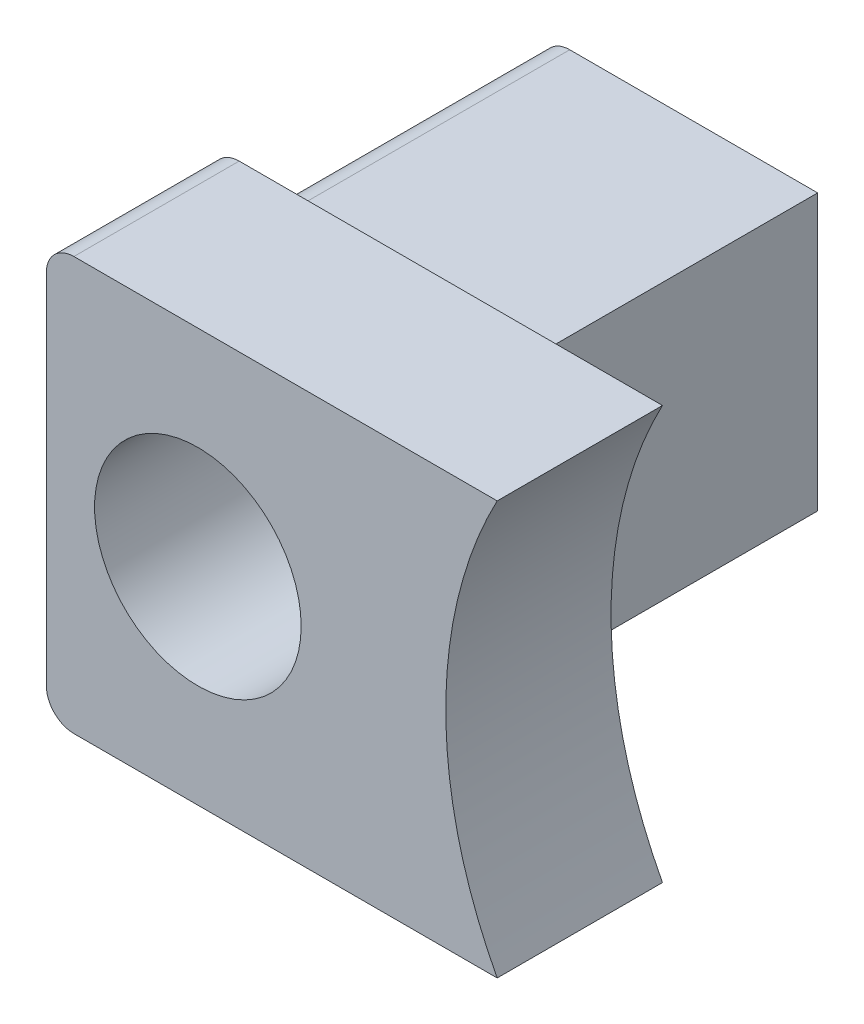
SolidWorks part; units mm, degrees
ref_plane "Front Plane" through (0, 0, 0) normal (0, 0, 1) x (1, 0, 0)
ref_plane "Top Plane" through (0, 0, 0) normal (0, 1, 0) x (1, 0, 0)
ref_plane "Right Plane" through (0, 0, 0) normal (1, 0, 0) x (0, 0, -1)
sketch "Sketch1" plane through (0, 0, 0) normal (0, 0, 1) x (1, 0, 0)
  line L1 (-8.25, 7.5) -> (8.25, 7.5)
  line L2 (-8.25, 7.5) -> (-8.25, -7.5)
  line L3 (-8.25, -7.5) -> (8.25, -7.5)
  line L4 (8.25, 7.5) -> (8.25, -7.5)
  line L5 (-8.25, 7.5) -> (8.25, -7.5) construction
  line L6 (-8.25, -7.5) -> (8.25, 7.5) construction
  point P0 (0, 0)
  dimension "D1" = 16.5
  dimension "D2" = 15
extrude "Boss-Extrude1" add sketch "Sketch1" along normal blind 18
fillet "Fillet1" radius 1 2 edges at (-8.25, -7.5, 9) (-8.25, 7.5, 9)
hole_wizard "CBORE for M4 Hex Socket Head Cap Screw1" positions "Sketch2" profile "Sketch3" counterbore size "M4" standard "ISO" end condition up to next
sketch "Sketch2" plane through (0, 0, 18) normal (0, 0, 1) x (1, 0, 0)
  line L0 (-8.25, 6.5) -> (-8.25, -6.5) construction
  point P0 (-2.75, 0)
  dimension "D1" = 5.5
sketch "Sketch3" plane through (-2.75, 0, 18) normal (1, 0, 0) x (0, -1, 0)
  line L0 (0, 0) -> (0, 18)
  line L1 (0, 18) -> (2.25, 18)
  line L3 (2.25, 18) -> (2.25, 8)
  line L4 (2.25, 8) -> (3.75, 8)
  line L5 (3.75, 8) -> (3.75, 0)
  line L7 (3.75, 0) -> (0, 0)
  line L11 (0, -6.35) -> (0, 107.95) construction
  dimension "通孔孔直径" = 4.5
  dimension "通孔孔深度" = 18
  dimension "柱形沉头孔直径" = 7.5
  dimension "柱形沉头孔深度" = 8
sketch "Sketch7" plane through (0, 0, 18) normal (0, 0, 1) x (1, 0, 0)
  line L0 (8.25, -7.5) -> (8.25, 7.5) construction
  circle A0 centre (22.25, 0) radius 16
  dimension "D1" = 32
  dimension "D2" = 14
extrude "Cut-Extrude2" cut sketch "Sketch7" against normal through all
sketch "Sketch8" plane through (0, 7.5, 0) normal (0, 1, 0) x (1, 0, 0)
  line L0 (8.1167, 0) -> (-7.25, 0) construction
  line L1 (1.75, 0) -> (8.25, 0)
  line L2 (1.75, 0) -> (1.75, -12)
  line L3 (1.75, -12) -> (8.25, -12)
  line L4 (8.25, 0) -> (8.25, -12)
  line L6 (-8.25, 0) -> (-8.25, -18) construction
  dimension "D1" = 12
  dimension "D2" = 10
extrude "Cut-Extrude3" cut sketch "Sketch8" against normal through all
sketch "Sketch9" plane through (0, -7.5, 0) normal (0, -1, 0) x (-1, 0, 0)
  line L0 (-1.75, 0) -> (-1.75, -12) construction
  line L1 (8.25, 0) -> (-1.75, 0)
  line L2 (8.25, 0) -> (8.25, -12)
  line L3 (8.25, -12) -> (-1.75, -12)
  line L4 (-1.75, 0) -> (-1.75, -12)
  line L5 (-1.75, -12) -> (-8.1167, -12) construction
extrude "Cut-Extrude4" cut sketch "Sketch9" against normal blind 2.5
mirror "Mirror1" about plane through (0, 0, 0) normal (0, 1, 0) of "Cut-Extrude4"
fillet "Fillet2" radius 1 2 edges at (-8.25, 5, 6) (-8.25, -5, 6)
